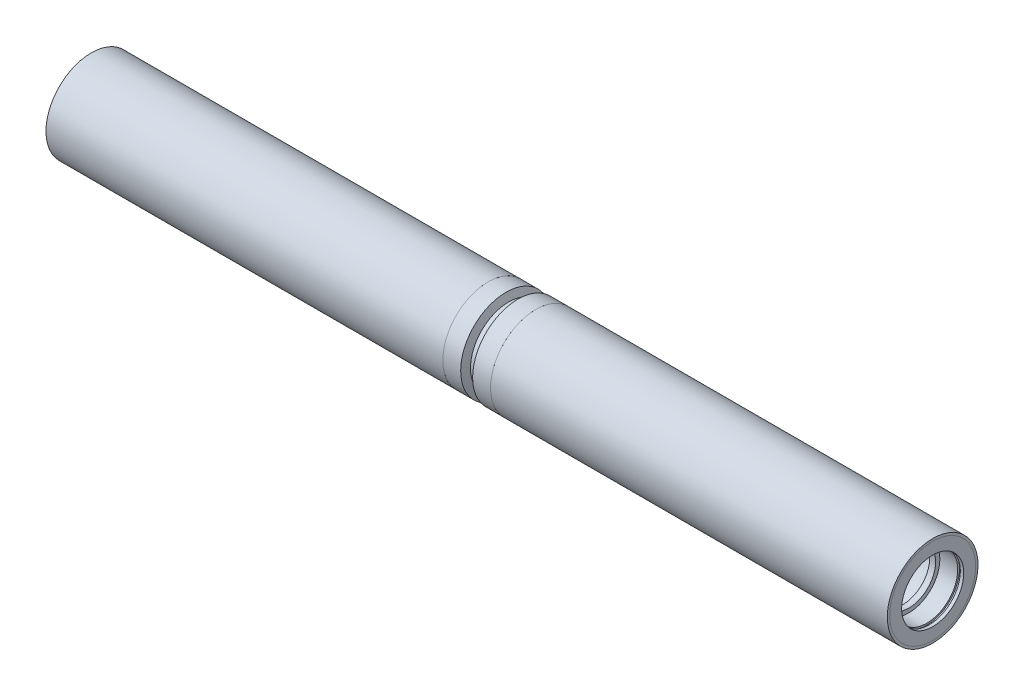
from build123d import *

# Parameters (mm, degrees)
SKETCH_1_W               = 705
SKETCH_1_H               = 2
SKETCH_2_R               = 36
SKETCH_2_R_2             = 22.5
EXTRUDE_1_DEPTH          = 25
SKETCH_3_R               = 36
SKETCH_3_R_2             = 22.5
EXTRUDE_2_DEPTH          = 25
CUT_EXTRUDE_1_DEPTH      = 357.572923818
CUT_EXTRUDE_1_DEPTH_BACK = 357.572923818
SKETCH_8_W               = 40
SKETCH_8_H               = 151.546664998


with BuildPart() as part:
    # 草图1 → 旋转1 (revolve)
    with BuildSketch(Plane.XY):
        with Locations((0, 37)):
            Rectangle(SKETCH_1_W, SKETCH_1_H)
    revolve(axis=Axis((0, 0, 0), (-1, 0, 0)))

    # 草图8 → 切除-拉伸1 (cut, two sides: drawn at the far end of the back side and taken through both)
    with BuildSketch(Plane.XY.offset(-CUT_EXTRUDE_1_DEPTH_BACK)):
        Rectangle(SKETCH_8_W, SKETCH_8_H)
    extrude(amount=CUT_EXTRUDE_1_DEPTH + CUT_EXTRUDE_1_DEPTH_BACK, mode=Mode.SUBTRACT)


with BuildPart() as body_2:
    # 草图2 → 凸台-拉伸1 (new body)
    with BuildSketch(Plane.ZY.offset(352.5)):
        with Locations(Location((0, 0, 0), (0, 0, 270))):
            Circle(SKETCH_2_R)
        with Locations(Location((0, 0, 0), (0, 0, 270))):
            Circle(SKETCH_2_R_2, mode=Mode.SUBTRACT)
    extrude(amount=-EXTRUDE_1_DEPTH)

    # 草图5 → 切除-旋转6 (revolve, cut)
    with BuildSketch(Plane.XY, mode=Mode.PRIVATE) as cut_revolve_6_sk:
        Polygon((-352.5, 26), (-349.7, 26), (-349.7, 27.5), (-347.5, 27.5), (-347.5, 26), (-332.5, 26), (-332.5, 0), (-352.5, 0), align=None)
    cut_revolve_6 = revolve(cut_revolve_6_sk.sketch.rotate(Axis((0, 0, 0), (-1, 0, 0)), 90), axis=Axis((0, 0, 0), (-1, 0, 0)), mode=Mode.SUBTRACT)


with BuildPart() as body_3:
    # 草图3 → 凸台-拉伸2 (new body)
    with BuildSketch(Plane(origin=(352.5, 0, 0), x_dir=(0, 0, -1), z_dir=(1, 0, 0))):
        with Locations(Location((0, 0, 0), (0, 0, 90))):
            Circle(SKETCH_3_R)
        with Locations(Location((0, 0, 0), (0, 0, 90))):
            Circle(SKETCH_3_R_2, mode=Mode.SUBTRACT)
    extrude(amount=-EXTRUDE_2_DEPTH)

    # 镜向2: 切除-旋转6 across plane
    add(cut_revolve_6.mirror(Plane(origin=(0, 0, 0), x_dir=(0, 0, 1), z_dir=(1, 0, 0))), mode=Mode.SUBTRACT)


with BuildPart() as cut_extrude_1_piece_1:
    # of the separate pieces the step leaves, piece 1, a body of its own (cut_extrude_1_pieces)
    add(part.part.solids().sort_by_distance((352.5, 36, 0))[0])


with BuildPart() as cut_extrude_1_piece_2:
    # of the separate pieces the step leaves, piece 2, a body of its own (cut_extrude_1_pieces)
    add(part.part.solids().sort_by_distance((-352.5, 36, 0))[0])


with BuildPart() as body_5:
    # 草图7 → 旋转2 (revolve)
    with BuildSketch(Plane.XY, mode=Mode.PRIVATE) as revolve_2_sk:
        Polygon((-30, -36), (-20, -36), (-20, -38), (20, -38), (20, -36), (30, -36), (30, -11), (-30, -11), align=None)
    revolve(revolve_2_sk.sketch.rotate(Axis((0, 0, 0), (1, 0, 0)), 270), axis=Axis((0, 0, 0), (1, 0, 0)))

    # 草图6 → 切除-旋转7 (revolve, cut)
    with BuildSketch(Plane.XY, mode=Mode.PRIVATE) as cut_revolve_7_sk:
        Polygon((-2.816178594, 32), (2.816178594, 32), (5, 38), (-5, 38), align=None)
    revolve(cut_revolve_7_sk.sketch.rotate(Axis((0, 0, 0), (-1, 0, 0)), 90), axis=Axis((0, 0, 0), (-1, 0, 0)), mode=Mode.SUBTRACT)


solid = Compound([body_2.part, body_3.part, cut_extrude_1_piece_1.part, cut_extrude_1_piece_2.part, body_5.part])
